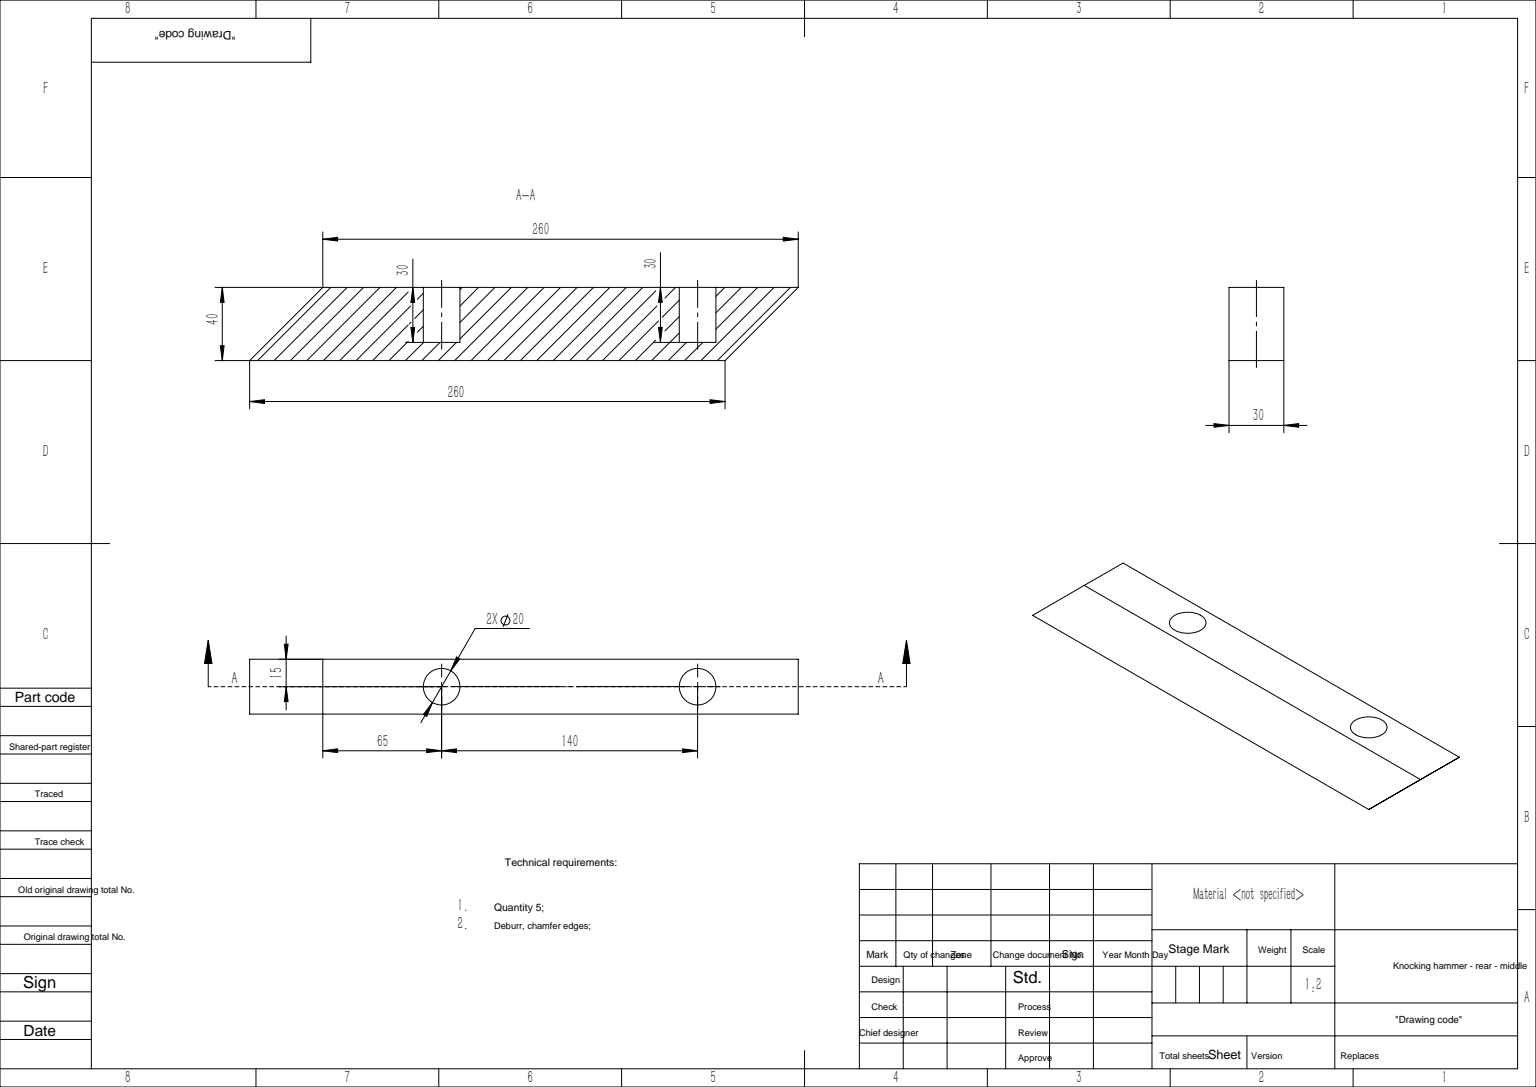
from build123d import *

# Parameters (mm, degrees)
SKETCH_1_W          = 270
SKETCH_1_H          = 30
EXTRUDE_1_DEPTH     = 40
SKETCH_2_R          = 10
CUT_EXTRUDE_2_DEPTH = 30
SKETCH_7_W          = 30
SKETCH_7_H          = 40
CUT_EXTRUDE_5_DEPTH = 10
CUT_EXTRUDE_6_DEPTH = 144.961800489
SKETCH_5_W          = 30
SKETCH_5_H          = 40
EXTRUDE_3_DEPTH     = 40
CUT_EXTRUDE_4_DEPTH = 183.002747232


with BuildPart() as part:
    # 草图1 → 凸台-拉伸1 (new body)
    with BuildSketch(Plane(origin=(0, 0, 0), x_dir=(1, 0, 0), z_dir=(0, 1, 0))):
        Rectangle(SKETCH_1_W, SKETCH_1_H)
    extrude(amount=EXTRUDE_1_DEPTH)

    # 草图2 → 切除-拉伸2 (cut)
    with BuildSketch(Plane(origin=(0, 40, 0), x_dir=(1, 0, 0), z_dir=(0, 1, 0))):
        with Locations(Location((70, 0, 0), (0, 0, 270))):
            Circle(SKETCH_2_R)
        with Locations(Location((-70, 0, 0), (0, 0, 90))):
            Circle(SKETCH_2_R)
    extrude(amount=-CUT_EXTRUDE_2_DEPTH, mode=Mode.SUBTRACT)

    # 草图7 → 切除-拉伸5 (cut)
    with BuildSketch(Plane(origin=(135, 0, 0), x_dir=(0, 0, -1), z_dir=(1, 0, 0))):
        with Locations((0, 20)):
            Rectangle(SKETCH_7_W, SKETCH_7_H)
    extrude(amount=-CUT_EXTRUDE_5_DEPTH, mode=Mode.SUBTRACT)

    # 草图8 → 切除-拉伸6 (cut, through all)
    with BuildSketch(Plane.XY.offset(15)):
        Polygon((125, 40), (85, 0), (125, 0), align=None)
    extrude(amount=-CUT_EXTRUDE_6_DEPTH, mode=Mode.SUBTRACT)

    # 草图5 → 凸台-拉伸3 (add)
    with BuildSketch(Plane.ZY.offset(135)):
        with Locations((0, 20)):
            Rectangle(SKETCH_5_W, SKETCH_5_H)
    extrude(amount=EXTRUDE_3_DEPTH)

    # 草图6 → 切除-拉伸4 (cut, through all)
    with BuildSketch(Plane.XY.offset(15)):
        Polygon((-175, 0), (-135, 40), (-175, 40), align=None)
    extrude(amount=-CUT_EXTRUDE_4_DEPTH, mode=Mode.SUBTRACT)


solid = part.part
